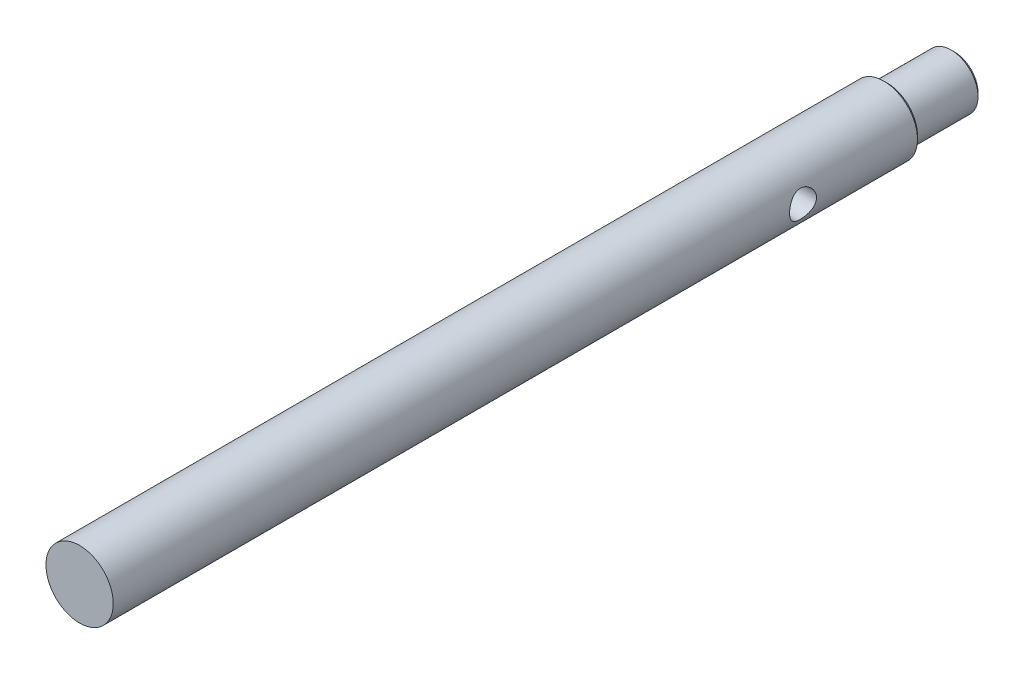
from build123d import *

# Parameters (mm, degrees)
SKETCH2_W               = 150
SKETCH2_H               = 10
CUT_EXTRUDE1_DEPTH      = 10
CUT_EXTRUDE1_DEPTH_BACK = 10
SKETCH5_R               = 4
BOSS_EXTRUDE3_START     = 70
SKETCH7_R               = 10
BOSS_EXTRUDE3_DEPTH     = 70
SKETCH3_R               = 10
BOSS_EXTRUDE4_DEPTH     = 20
SKETCH8_R               = 8
BOSS_EXTRUDE5_DEPTH     = 20
CHAMFER1_SIZE           = 1
CHAMFER2_SIZE           = 1


with BuildPart() as part:
    # Sketch2 → Revolve4 (revolve)
    with BuildSketch(Plane(origin=(0, 0, 0), x_dir=(0, 0, -1), z_dir=(1, 0, 0)), mode=Mode.PRIVATE) as revolve4_sk:
        with Locations((75, 5)):
            Rectangle(SKETCH2_W, SKETCH2_H)
    revolve(revolve4_sk.sketch.rotate(Axis((0, 0, 0), (0, 0, -1)), 90), axis=Axis((0, 0, 0), (0, 0, -1)))

    # Sketch5 → Cut-Extrude1 (cut, two sides: drawn at the far end of the back side and taken through both)
    with BuildSketch(Plane(origin=(0, 0, 0), x_dir=(0, 0, -1), z_dir=(1, 0, 0)).offset(-CUT_EXTRUDE1_DEPTH_BACK)):
        with Locations(Location((135, 0, 0), (0, 0, 180))):
            Circle(SKETCH5_R)
    extrude(amount=CUT_EXTRUDE1_DEPTH + CUT_EXTRUDE1_DEPTH_BACK, mode=Mode.SUBTRACT)

    # Sketch7 → Boss-Extrude3 (add)
    with BuildSketch(Plane.XY.offset(BOSS_EXTRUDE3_START)):
        Circle(SKETCH7_R)
    extrude(amount=-BOSS_EXTRUDE3_DEPTH)

    # Sketch3 → Boss-Extrude4 (add)
    with BuildSketch(Plane(origin=(0, 0, -150), x_dir=(-1, 0, 0), z_dir=(0, 0, -1))):
        with Locations(Location((0, 0, 0), (0, 0, 180))):
            Circle(SKETCH3_R)
    extrude(amount=BOSS_EXTRUDE4_DEPTH)

    # Sketch8 → Boss-Extrude5 (add)
    with BuildSketch(Plane(origin=(0, 0, -170), x_dir=(-1, 0, 0), z_dir=(0, 0, -1))):
        Circle(SKETCH8_R)
    extrude(amount=BOSS_EXTRUDE5_DEPTH)

    # Chamfer1
    chamfer1_edges = [part.edges().sort_by_distance(p)[0] for p in [
        (8, 0, -190),
    ]]
    chamfer(chamfer1_edges, length=CHAMFER1_SIZE)

    # Chamfer2
    chamfer2_edges = [part.edges().sort_by_distance(p)[0] for p in [
        (-10, 0, -170),
    ]]
    chamfer(chamfer2_edges, length=CHAMFER2_SIZE)


solid = part.part
